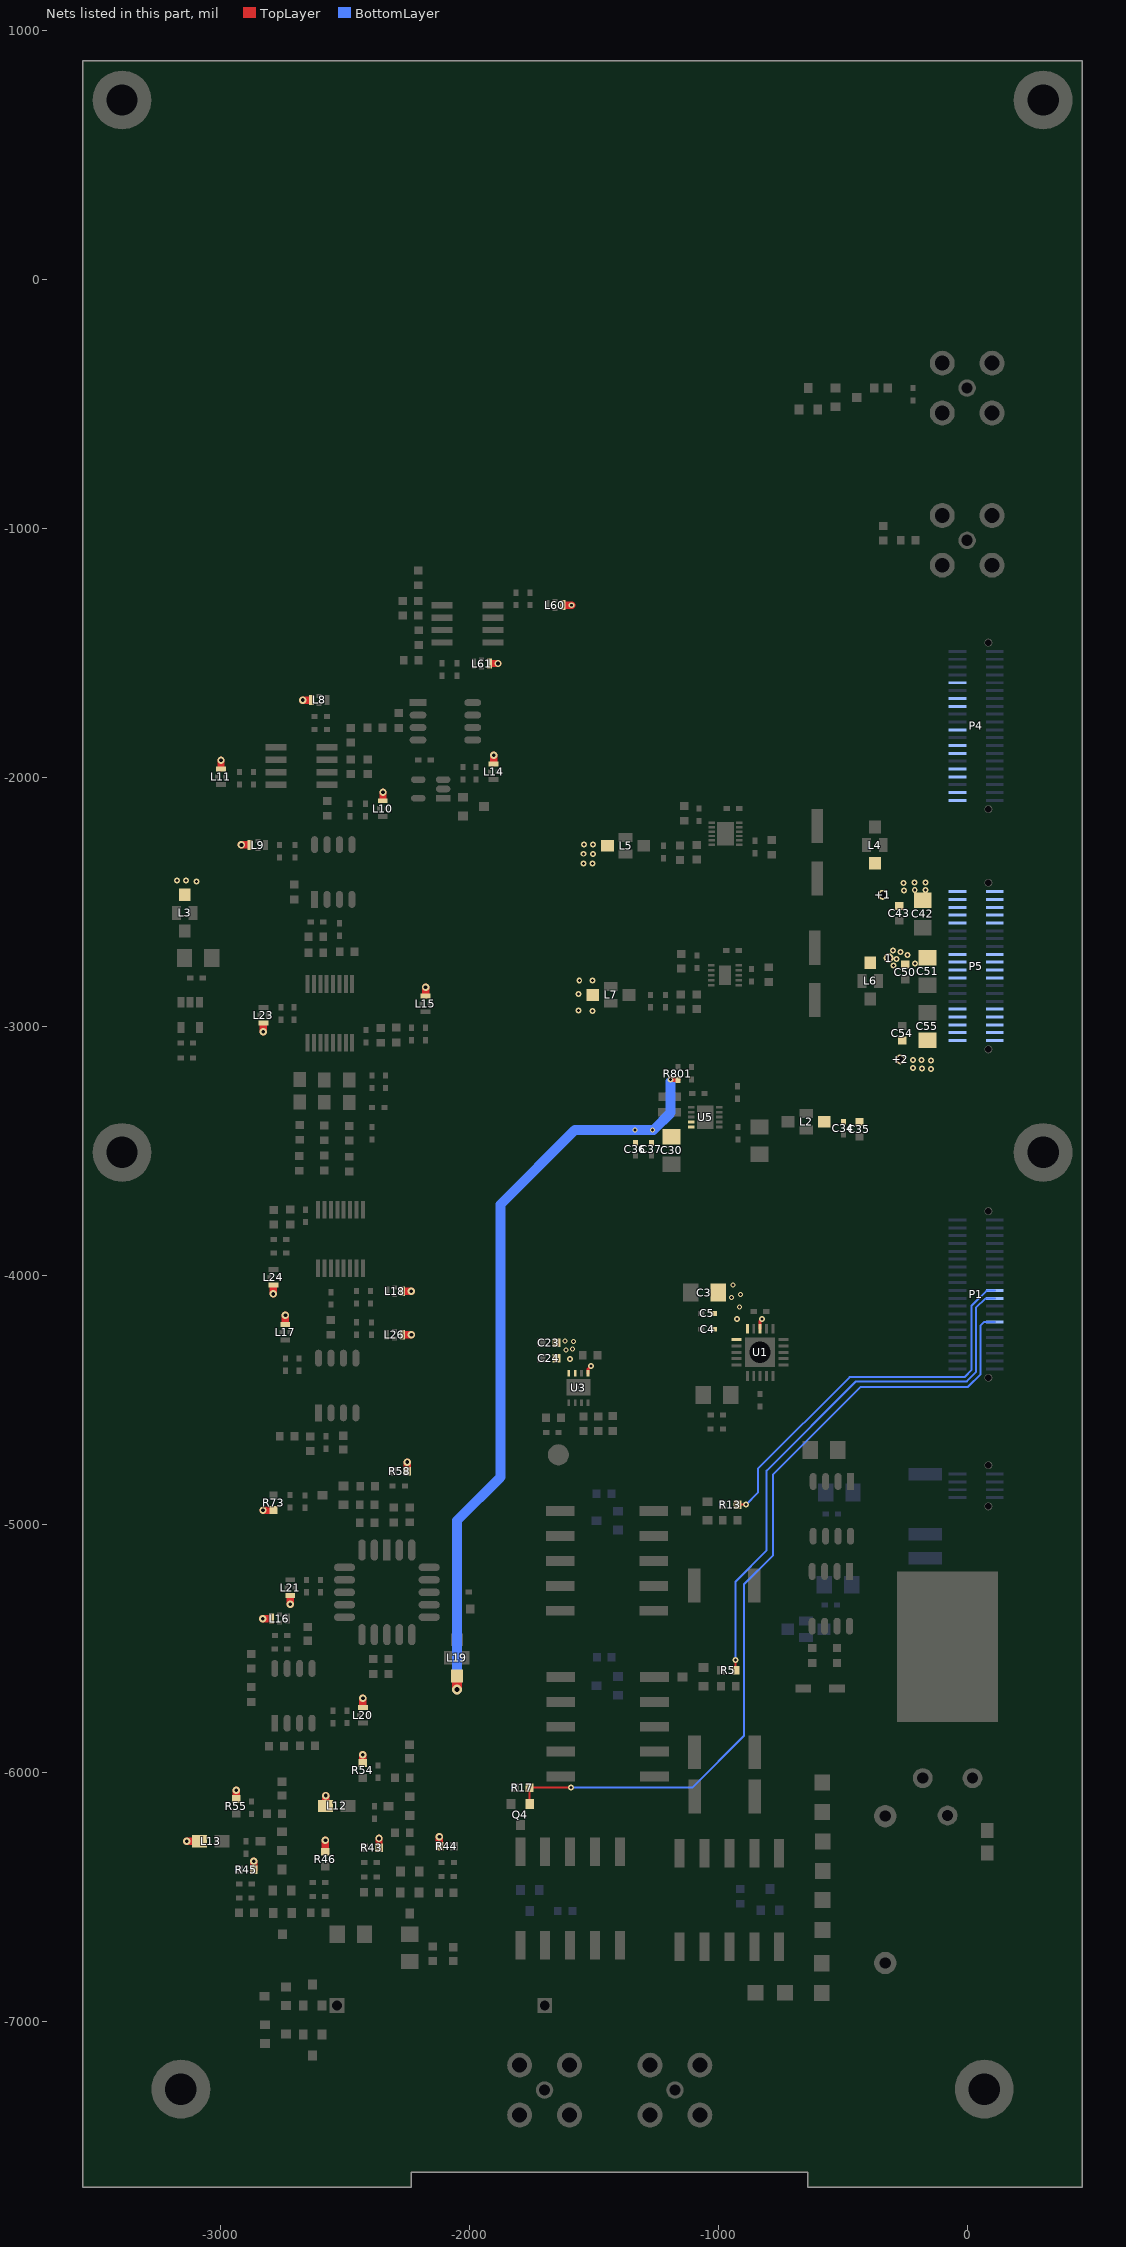
[diagram p0: the nets of this part, all layers, seen from the top]
# Altium PCB MISC109358.PcbDoc (part 2 of 7)
Units mil, origin at the board's own origin, x right, y up, seen from the top; angles counter-clockwise.
Board outline 4015.75 x 8543.31 mil, 4 copper layers (TopLayer, GND, POWER, BottomLayer), stack 33.234 mil thick; 299 components, 170 nets, 998 pads, 2318 vias.

## Part data
1 +1 +2: library part TP
C3 C4 C5 C6 C7 C8 C9 C14 C15 C16 C17 C18 C20 C21 C28 C29 C30 C31 C32 C33 C34 C35 C36 C37 C38 C39 C40 C41 C42 C43 C46 C47 C50 C51 C53 C54 C55 C57 C58 C60 C63 C66 C67 C68 C69 C70 C72 C73 C74 C75 C76 C77 C78 C79 C80 C81 C82 C83 C84 C85 C86 C89 C90 C91 C92 C93 C94 C96 C97 C98 C99 C100 C101 C102 C103 C104 C105 C106 C107 C108 C110 C111 C112 C114 C115 C116 C117 C118 C119 C120 C121 C122 C123 C124 C125 C126 C127 C128 C129 C301 C302 C304 C305 C306 C307: library part CAP, "Capacitor"
C22 C23 C25 C26 C45 C48 C59 C61 C64 C65 C334: library part C1206
C24 C27: library part C0402
C49 C62: library part CAPACITOR_1, "Capacitor"
C56 C71 C87 C88 C95 C109 C113: library part CAPACITOR, "Capacitor"
D1 D4 D6 D7: library part DIODE, "Diode"
D5 D10: library part ZENER3, "Zener Diode"
D11: library part MMBZ5257BLT1G
J1 J2 P6 P9: library part JA1
K1 K2 K3 K4: library part TQ2SS-5V
L8 L9 L10 L11 L14 L15 L16 L17 L18 L20 L21 L23 L24 L26 L60 L61: library part NFM15PC104R1A3D
L12 L13 L22 L25 L27: library part INDUCTOR
P1 P4 P5: "Header, 20-Pin, Dual row"
P2: "Header, 4-Pin, Dual row"
Q1 Q3 Q15 Q16: library part NPN, "NPN Transistor"
Q7 Q8 Q9 Q10 Q11 Q12: library part D1, "Diode"
Q13 Q14: library part MMBZ5231B
Q17: library part PNP, "PNP Transistor"
R1 R20 R33 R68 R72: library part RES
R2 R3 R4 R5 R6 R7 R8 R9 R10 R12 R13 R14 R16 R17 R18 R19 R21 R22 R23 R24 R25 R26 R27 R28 R29 R30 R31 R32 R34 R35 R36 R37 R38 R39 R40 R41 R42 R43 R44 R45 R46 R47 R48 R49 R50 R51 R52 R53 R54 R55 R56 R57 R58 R59 R60 R61 R62 R63 R64 R65 R66 R67 R69 R70 R71 R73 R74 R75 R76 R77 R78 R79 R800 R801: library part RES1
R11 R15: library part R0603
TP1: library part TEST_2
U1: library part TPS7A4701RGWR(QFN20)
U2 U4: library part TC4426COA
U3: "3PEAK"
U6: library part ADR391AUJZ-REEL7
U11 U60: library part AD8002ARZ
U13: library part DG540DN
U14: library part LMH6624MA

## Free pads (board coordinates)
  round 236.22 hole 125.98: 0(-3159.3,-7270.3) 0(69.05,-7270.3) 2(305.27,721.83) 3(-3395.52,-3506.52) 3(-3395.52,721.83) 3(305.27,-3506.52)

## Via types
v1: diameter 24, hole 12, TopLayer to BottomLayer, 2184 vias
v2: diameter 20, hole 12, TopLayer to BottomLayer, 95 vias
v3: diameter 30, hole 15, TopLayer to BottomLayer, 37 vias
v4: diameter 40, hole 20, TopLayer to BottomLayer, 2 vias

## Nets (pads, with @x,y where several pads share a name; then routed paths per layer and width w, separated by ;. In a path a pad name is that pad's centre, name@x,y a point inside that pad or via, vN(x,y) a via of type N, cw(c..) or ccw(c..) an arc to the next point about the centre after c; other vN are vias at no path point)
12.4V: +2.1 C3.1 C4.1 C5.1 C34.1 C35.1 C54.1 C55.1 L2.3 P5.31 P5.32 P5.33 P5.34 P5.35 P5.36 P5.37 P5.38 P5.39 P5.40 U1.13 U1.15 U1.16 | length 41.9
  TopLayer w12: U1.13@-831.82,-4215.02 -831.82,-4184.82 v1(-823.52,-4176.52)
  other v1: -925.52,-4176.52 -144.52,-3171.52 -180.52,-3169.52 -217,-3167.52 -145.52,-3136.52 -182.52,-3135.52 -217,-3134.52
  other v2: -914.52,-4128.52 -946.52,-4089.52 -910.52,-4076.52 -940.52,-4038.52
+5V: L3.1 L7.3 L8.3 L9.1 L12.1 L13.1 L15.1 L16.1 L17.1 L24.3 L60.3 R44.1 R46.1 R58.1 | length 416.5
  TopLayer w30: v3(-3135.52,-6274.52) L13.1@-3083.52,-6274.52 ; v3(-2916.04,-2271.04) L9.1@-2886.64,-2271.04 ; v3(-2830.66,-5380.52) L16.1@-2800.52,-5380.52 ; v3(-2788,-4075.04) L24.3@-2788,-4045.64 ; L17.1@-2739.04,-4190.39 v3(-2739.04,-4161) ; v3(-2670.04,-1689.04) L8.3@-2640.64,-1689.04 ; R46.1@-2578.52,-6312.52 v3(-2578.52,-6270.52) ; L12.1@-2577.52,-6132.52 v3(-2577.52,-6090.52) ; R58.1@-2249.52,-4787.52 v3(-2249.52,-4750.52) ; L15.1@-2176.04,-2872.39 v3(-2176.04,-2843) ; R44.1@-2120.52,-6293.52 v3(-2120.52,-6256.52) ; L60.3@-1618.39,-1308 v1(-1589,-1308)
  other v1: -1504.52,-2937.52 -1562.1,-2935.52 -1562.1,-2869.52 -1558.52,-2815.52 -1505.52,-2815.52 -3095.52,-2418.52 -3175.52,-2414.52 -3138.52,-2414.52
-5.4V: +1.1 C42.1 C43.1 L4.1 P5.1 P5.2 P5.3 P5.4 P5.5 P5.6 P5.7 P5.8 P5.9 P5.10
  other v1: -254.52,-2454.52 -210.52,-2451.52 -167.52,-2451.52 -255.52,-2423.52 -211.52,-2422.52 -166.52,-2421.52
-5V: L5.3 L10.1 L11.3 L14.1 L18.3 L20.3 L21.1 L23.1 L26.1 L61.3 R43.2 R45.1 R54.2 R55.1 R73.2 | length 448.2
  TopLayer w30: L11.3@-2998.04,-1960.39 v3(-2998.04,-1931) ; R55.1@-2936.52,-6104.48 v3(-2936.52,-6069.52) ; R45.1@-2866.52,-6389.52 v3(-2866.52,-6354.94) ; v3(-2829.23,-4943.81) R73.2@-2787,-4943.81 ; v3(-2828,-3022.04) L23.1@-2828,-2992.64 ; v3(-2719.52,-5321.66) L21.1@-2719.52,-5291.52 ; R54.2@-2428.52,-5960.17 v3(-2428.52,-5926.52) ; L20.3@-2427.52,-5729.52 v3(-2427.52,-5699.38) ; R43.2@-2363.21,-6299.52 v3(-2363.21,-6262.83) ; L10.1@-2347.04,-2088.39 v3(-2347.04,-2059) ; L18.3@-2263.39,-4063.94 v3(-2234,-4063.94) ; L26.1@-2262.39,-4239 v3(-2233,-4239) ; L61.3@-1914.39,-1542 v3(-1885,-1542) ; L14.1@-1902.04,-1940.16 v3(-1902.04,-1910.76)
  other v1: -1541.52,-2345.52 -1504.52,-2345.52 -1541.48,-2306.52 -1502.52,-2306.76 -1503.52,-2269.49 -1539.52,-2268.52
A6V: 1.1 C23.2 C24.1 C50.2 C51.1 L6.1 P5.17 P5.18 P5.19 P5.20 P5.21 P5.22 P5.23 P5.24 U3.5 U3.7 U3.8 | length 33.3
  TopLayer w11: U3.5@-1523.71,-4393.81 -1523.71,-4377.71 v1(-1511.52,-4365.52)
  other v1: -1596.52,-4336.52 -296.52,-2755.52 -209.52,-2746.52 -283.52,-2729.52 -239.52,-2713.52 -268.52,-2701.52 -298.52,-2695.52
  other v2: -1612.52,-4300.52 -1585.52,-4295.52 -1582.52,-4265.52 -1616.52,-4263.52
A12V: C30.1 C36.1 C37.1 L19.3 R801.1 U5.9 U5.10 | length 3068.7
  TopLayer w20: v1(-1191.48,-3214.52) R801.1@-1162.48,-3214.52
  TopLayer w40: v4(-2050.04,-5665) L19.3@-2050.04,-5610.19
  BottomLayer w40: v4(-2050.04,-5665) -2050.04,-4986.04 -1875.52,-4811.52 -1875.52,-3715.52 -1576.52,-3416.52 v2(-1334.64,-3416.52) v2(-1264.52,-3416.52) -1260.52,-3416.52 -1191,-3347 v1@-1191,-3221
AK1: P1.27 Q4.1 R17.2 | length 3370.9
  TopLayer w8: Q4.1@-1757.73,-6124.31 R17.2@-1757.73,-6058.52 v1(-1592.52,-6058.52)
  BottomLayer w8: v1(-1592.52,-6058.52) -1104.52,-6058.52 -896.52,-5850.52 -896.52,-5242.52 -780.52,-5126.52 -780.52,-4801.52 -427.52,-4448.52 3.48,-4448.52 54.48,-4397.52 54.48,-4201.52 68.55,-4187.45 P1.27@111.04,-4187.45
AK10: P1.19 R13.2 | length 1598.1
  TopLayer w8: R13.2@-922.83,-4921.52 v1(-888.52,-4921.52)
  BottomLayer w8: v1(-888.52,-4921.52) -840.52,-4873.52 -840.52,-4777.52 -472.52,-4409.52 -10.52,-4409.52 18.48,-4380.52 18.48,-4121.52 78.54,-4061.46 P1.19@111.04,-4061.46
AK13: P1.21 R5.2 | length 2207.5
  TopLayer w8: R5.2@-930.52,-5586.69 v1(-930.52,-5545.52)
  BottomLayer w8: v1(-930.52,-5545.52) -930.52,-5230.52 -805.52,-5105.52 -805.52,-4785.52 -446.52,-4426.52 -1.52,-4426.52 35.48,-4389.52 35.48,-4131.52 74.04,-4092.96 P1.21@111.04,-4092.96
AS27: P4.38
AS28: P4.40
ATTN1: P4.34
ATTN2: P4.32
ATTN4: P4.28
ATTN8: P4.26
ATTN16: P4.22
"DAC CLK": P4.14
"DAC DATA": P4.16
"DAC STROBE": P4.10